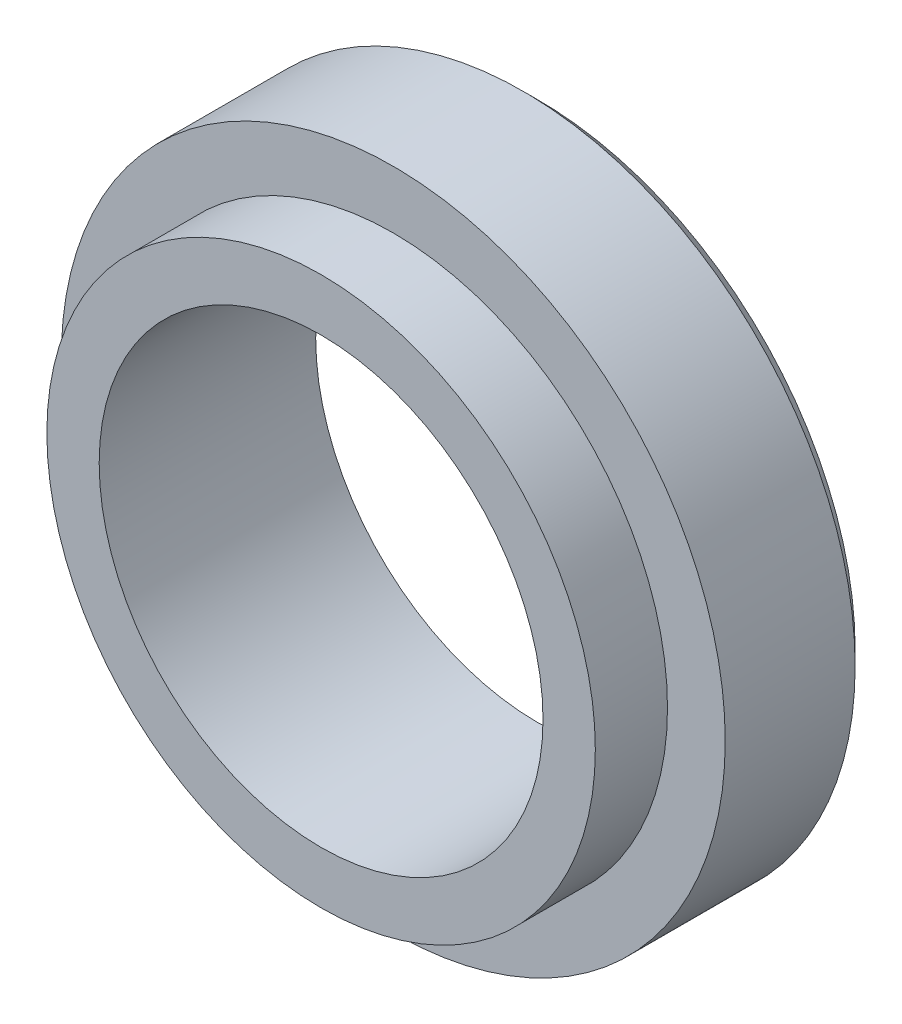
SolidWorks part; units mm, degrees
material "Q235"
ref_plane "Front Plane" through (0, 0, 0) normal (0, 0, 1) x (1, 0, 0)
ref_plane "Top Plane" through (0, 0, 0) normal (0, 1, 0) x (1, 0, 0)
ref_plane "Right Plane" through (0, 0, 0) normal (1, 0, 0) x (0, 0, -1)
sketch "Sketch1" plane through (0, 0, 0) normal (0, 0, 1) x (1, 0, 0)
  circle A0 centre (0, 0) radius 19
  circle A1 centre (0, 0) radius 7.5
  dimension "D1" = 38
  dimension "D2" = 15
extrude "Boss-Extrude1" add sketch "Sketch1" along normal blind 10
sketch "Sketch2" plane through (0, 0, 10) normal (0, 0, 1) x (1, 0, 0)
  circle A0 centre (0, 0) radius 7.5 construction
  circle A1 centre (0, 0) radius 7.5
  circle A2 centre (0, 0) radius 23
  dimension "D1" = 46
extrude "Boss-Extrude2" add sketch "Sketch2" along normal blind 10
sketch "Sketch3" plane through (0, 0, 20) normal (0, 0, 1) x (1, 0, 0)
  circle A0 centre (0, 0) radius 7.5 construction
  circle A1 centre (0, 0) radius 7.5
  circle A2 centre (0, 0) radius 19 construction
  circle A3 centre (0, 0) radius 19
extrude "Boss-Extrude3" add sketch "Sketch3" along normal blind 5
hole_wizard "G1 Tapped Hole1" positions "Sketch4" profile "Sketch5" tap size "G1" standard "GB"
sketch "Sketch4" plane through (0, 0, 25) normal (0, 0, 1) x (1, 0, 0)
  point P0 (0, 0)
sketch "Sketch5" plane through (0, 0, 25) normal (1, 0, 0) x (0, -1, 0)
  line L0 (0, 0) -> (0, 82.6682)
  line L1 (0, 82.6682) -> (15.375, 73.43)
  line L2 (15.375, 73.43) -> (15.375, 0)
  line L5 (15.375, 0) -> (0, 0)
  line L10 (0, 82.6682) -> (-15.375, 73.43) construction
  line L11 (0, -6.35) -> (0, 107.95) construction
  dimension "螺纹孔钻头直径" = 30.75
  dimension "螺纹孔钻头深度" = 73.43
  dimension "导头角度" = 118
cosmetic thread "Hole cosmetic thread1" parameters "D1"=15, "D2"=33.249
sketch "Sketch6" plane through (0, 0, 0) normal (0, 0, 1) x (1, 0, 0)
  circle A0 centre (0, 0) radius 28.4739
extrude "Cut-Extrude1" cut sketch "Sketch6" along normal blind 10
chamfer "Chamfer2" distance 1 angle 45 1 edges at (23, 0, 10)
